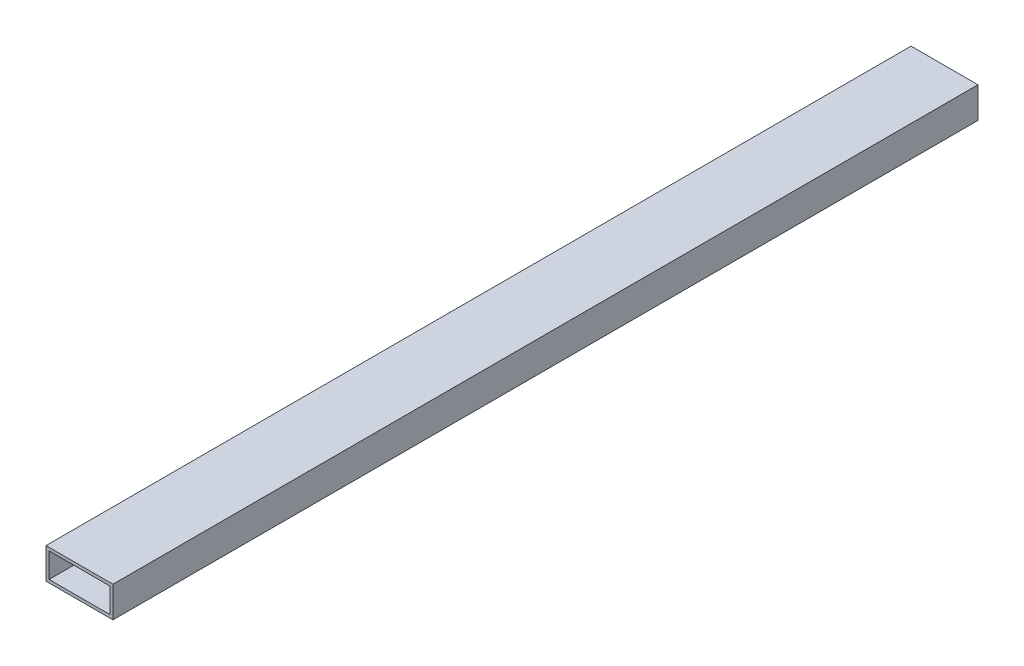
SolidWorks part; units mm, degrees
ref_plane "Front Plane" through (0, 0, 0) normal (0, 0, 1) x (1, 0, 0)
ref_plane "Top Plane" through (0, 0, 0) normal (0, 1, 0) x (1, 0, 0)
ref_plane "Right Plane" through (0, 0, 0) normal (1, 0, 0) x (0, 0, -1)
other "Configuration Table"
sketch "Sketch1" plane through (0, 0, 0) normal (0, 0, 1) x (1, 0, 0)
  line L0 (-40.5408, 39.808) -> (24.4592, 39.808)
  line L1 (24.4592, 39.808) -> (24.4592, 9.808)
  line L2 (24.4592, 9.808) -> (-40.5408, 9.808)
  line L3 (-40.5408, 9.808) -> (-40.5408, 39.808)
extrude "Boss-Extrude1" add sketch "Sketch1" along normal blind 840
sketch "Sketch2" plane through (0, 0, 840) normal (0, 0, 1) x (1, 0, 0)
  line L0 (-37.5408, 36.808) -> (21.4592, 36.808)
  line L1 (21.4592, 36.808) -> (21.4592, 12.808)
  line L2 (21.4592, 12.808) -> (-37.5408, 12.808)
  line L3 (-37.5408, 12.808) -> (-37.5408, 36.808)
  line L4 (24.4592, 39.808) -> (-40.5408, 39.808) construction
  line L5 (24.4592, 9.808) -> (24.4592, 39.808) construction
  line L6 (-40.5408, 9.808) -> (24.4592, 9.808) construction
  line L7 (-40.5408, 39.808) -> (-40.5408, 9.808) construction
  dimension "D1" = 3
  dimension "D2" = 3
  dimension "D3" = 3
  dimension "D4" = 3
extrude "Cut-Extrude1" cut sketch "Sketch2" against normal blind 950
sketch "Sketch3" plane through (0, 39.808, 0) normal (0, 1, 0) x (1, 0, 0)
  line L0 (-8.0408, 0) -> (-8.0408, -39.0581) construction
  line L1 (24.4592, 0) -> (-40.5408, 0) construction
  circle A0 centre (-8.0408, -39.0581) radius 9.584
